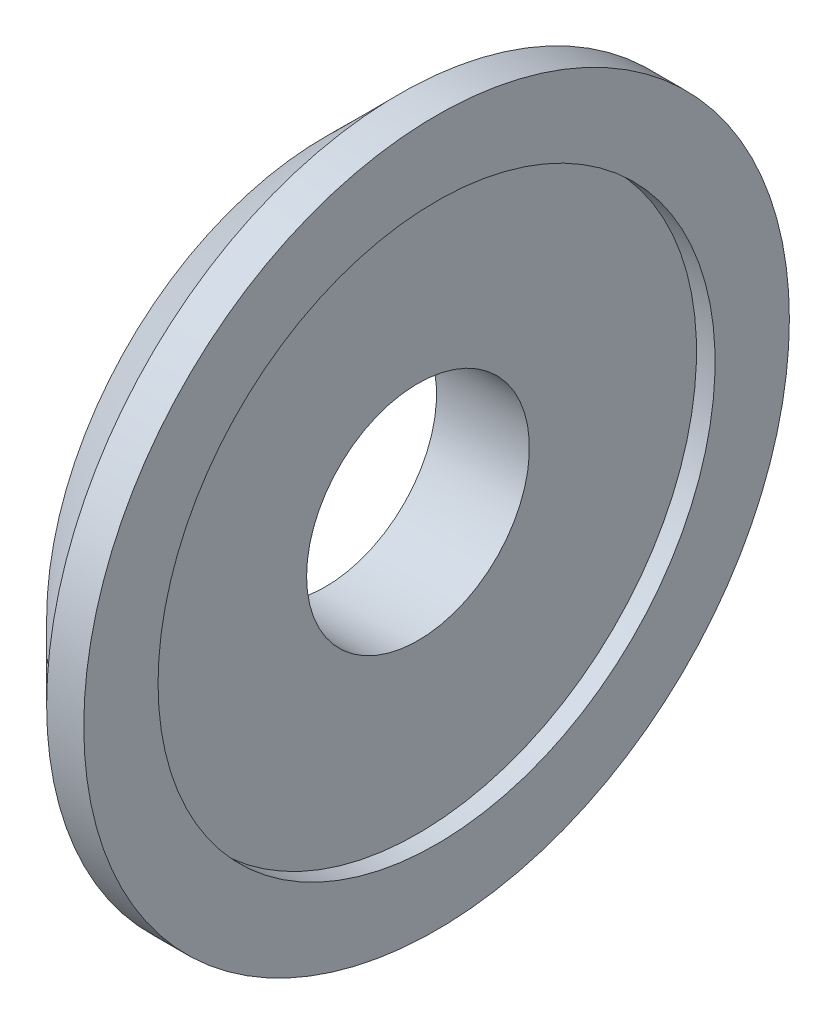
from build123d import *


with BuildPart() as part:
    # Sketch1 → Revolve2 (revolve)
    with BuildSketch(Plane.XY, mode=Mode.PRIVATE) as revolve2_sk:
        Polygon((-3, 15), (-3, 6), (2, 6), (2, 15), (3, 15), (3, 19), (1, 19), align=None)
    revolve(revolve2_sk.sketch.rotate(Axis((-11.259866943, 0, 0), (1, 0, 0)), 90), axis=Axis((-11.259866943, 0, 0), (1, 0, 0)))


solid = part.part
